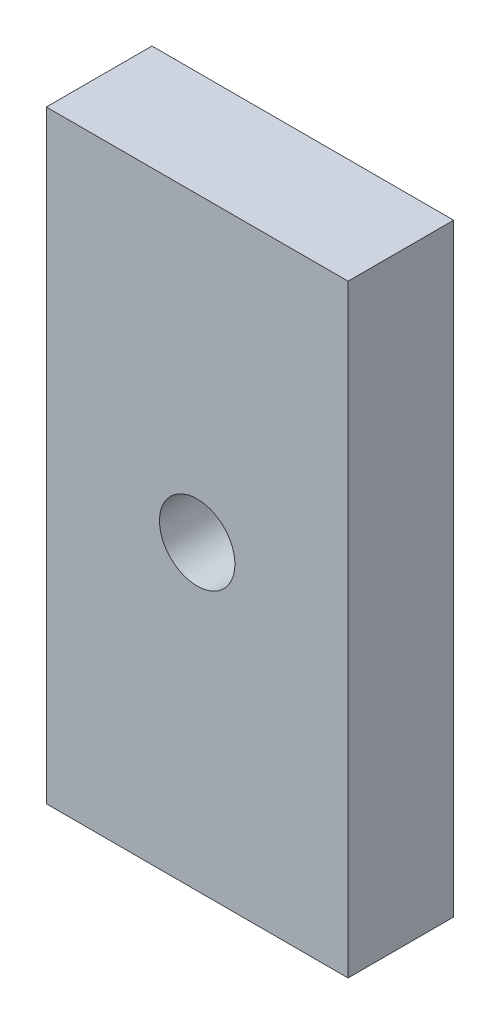
from build123d import *

# Parameters (mm, degrees)
SKETCH1_W           = 40
SKETCH1_H           = 80
SKETCH1_R           = 5
BOSS_EXTRUDE1_DEPTH = 14


with BuildPart() as part:
    # Sketch1 → Boss-Extrude1 (new body)
    with BuildSketch(Plane.XY):
        with Locations((20, 40)):
            Rectangle(SKETCH1_W, SKETCH1_H)
        with Locations((20, 40)):
            Circle(SKETCH1_R, mode=Mode.SUBTRACT)
    extrude(amount=BOSS_EXTRUDE1_DEPTH)


solid = part.part
